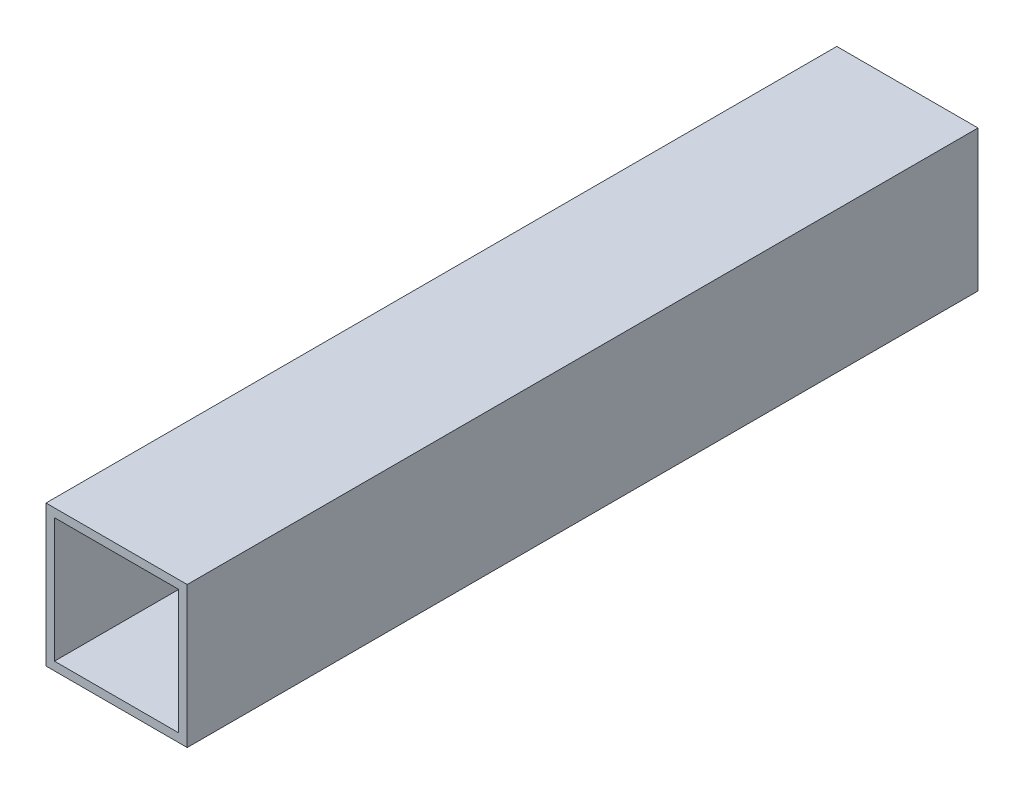
SolidWorks part; units mm, degrees
ref_plane "前视基准面" through (0, 0, 0) normal (0, 0, 1) x (1, 0, 0)
ref_plane "上视基准面" through (0, 0, 0) normal (0, 1, 0) x (1, 0, 0)
ref_plane "右视基准面" through (0, 0, 0) normal (1, 0, 0) x (0, 0, -1)
sketch "草图1" plane through (0, 0, 0) normal (0, 0, 1) x (1, 0, 0)
  line L0 (0, 0) -> (0, 50)
  line L1 (0, 50) -> (50, 50)
  line L2 (50, 50) -> (50, 0)
  line L3 (50, 0) -> (0, 0)
  line L4 (3, 3) -> (3, 47)
  line L5 (3, 47) -> (47, 47)
  line L6 (47, 47) -> (47, 3)
  line L7 (47, 3) -> (3, 3)
  dimension "D1" = 3
extrude "凸台-拉伸2" add sketch "草图1" along normal blind 280
